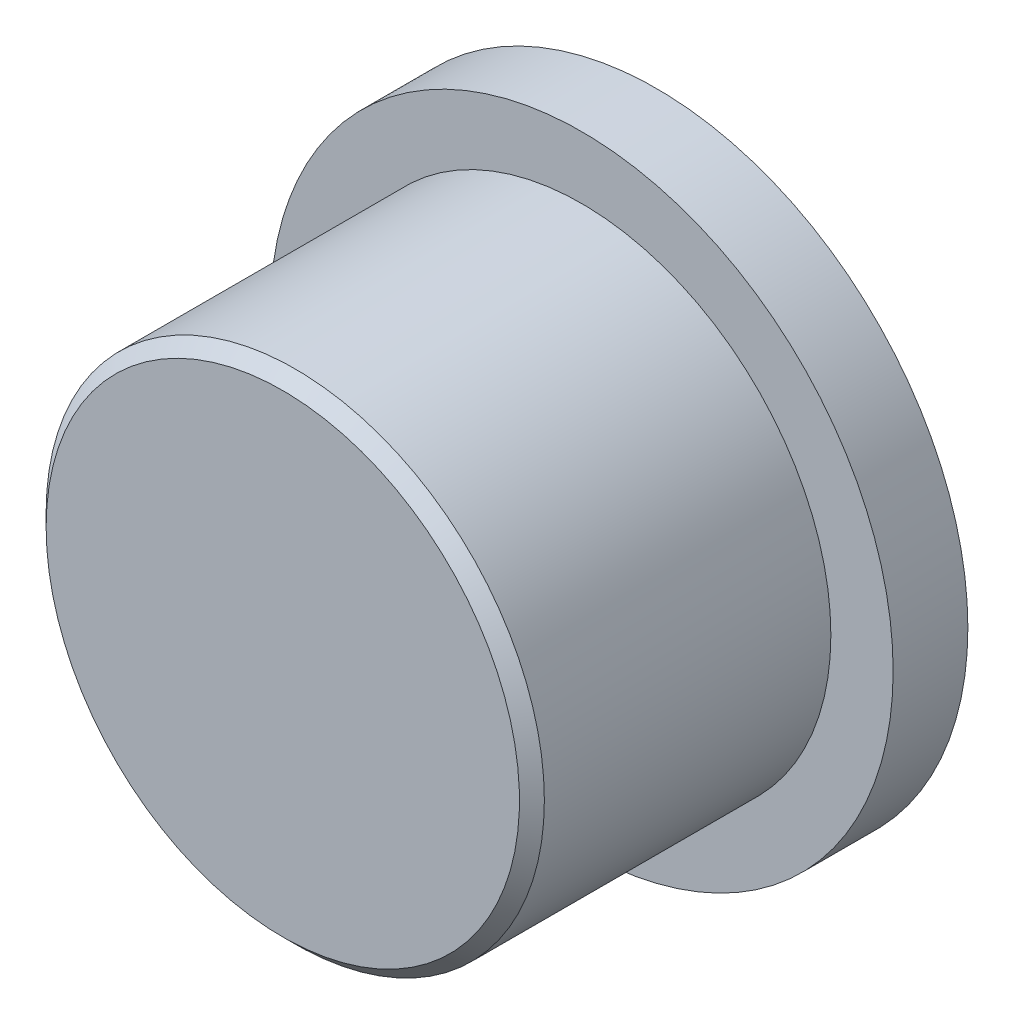
SolidWorks part; units mm, degrees
material "20#"
ref_plane "Front Plane" through (0, 0, 0) normal (0, 0, 1) x (1, 0, 0)
ref_plane "Top Plane" through (0, 0, 0) normal (0, 1, 0) x (1, 0, 0)
ref_plane "Right Plane" through (0, 0, 0) normal (1, 0, 0) x (0, 0, -1)
sketch "Sketch1" plane through (0, 0, 0) normal (1, 0, 0) x (0, 0, -1)
  line L0 (0, 0) -> (15, 0) construction
  line L1 (15, 0) -> (15, 12.5)
  line L2 (15, 12.5) -> (12, 12.5)
  line L3 (12, 12.5) -> (12, 10)
  line L4 (12, 10) -> (0, 10)
  line L5 (0, 10) -> (0, 0)
  line L6 (0, 0) -> (15, 0)
  dimension "D1" = 20
  dimension "D2" = 12
  dimension "D3" = 3
  dimension "D4" = 25
revolve "Revolve1" add sketch "Sketch1" angle 360 about L0
chamfer "Chamfer1" distance 0.5 angle 45 1 edges at (10, 0, 0)
